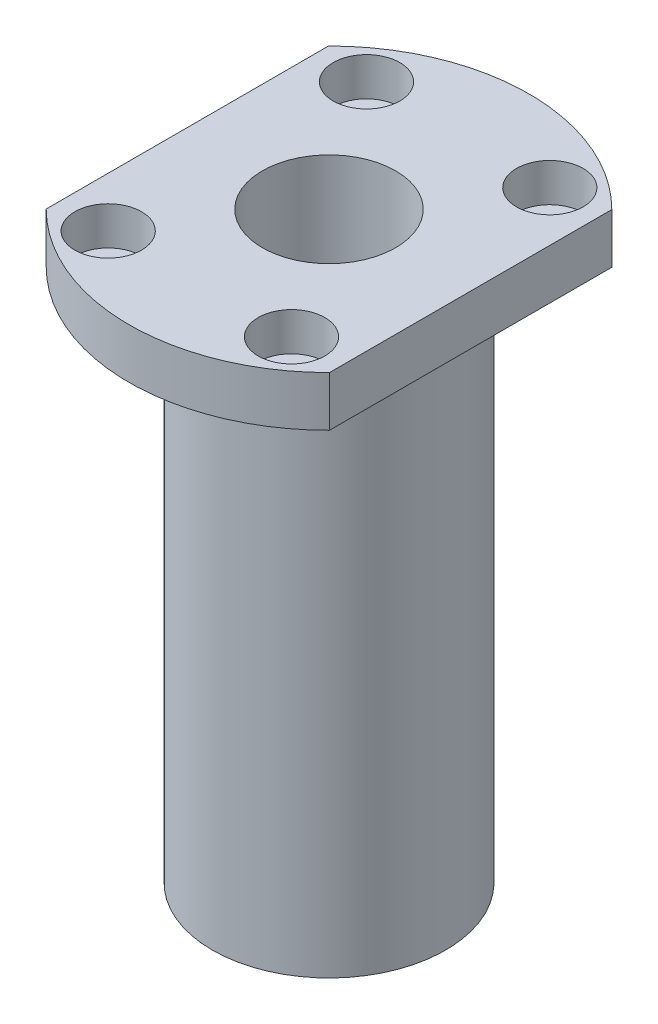
SolidWorks part; units mm, degrees
material "SS400"
ref_plane "Front Plane" through (0, 0, 0) normal (0, 0, 1) x (1, 0, 0)
ref_plane "Top Plane" through (0, 0, 0) normal (0, 1, 0) x (1, 0, 0)
ref_plane "Right Plane" through (0, 0, 0) normal (1, 0, 0) x (0, 0, -1)
sketch "Sketch1" plane through (0, 0, 0) normal (0, 1, 0) x (1, 0, 0)
  circle A0 centre (0, 0) radius 14
  dimension "D1" = 28
extrude "Boss-Extrude1" add sketch "Sketch1" along normal blind 64
sketch "Sketch2" plane through (0, 64, 0) normal (0, 1, 0) x (1, 0, 0)
  circle A0 centre (0, 0) radius 24
  dimension "D1" = 48
extrude "Boss-Extrude2" add sketch "Sketch2" along normal blind 6
sketch "Sketch3" plane through (0, 70, 0) normal (0, 1, 0) x (1, 0, 0)
  line L0 (0, 0) -> (0, 6.8507) construction
  line L1 (-17, 16.9411) -> (-17, -16.9411)
  line L2 (17, 16.9411) -> (17, -16.9411)
  arc A0 (17, 16.9411) -> (-17, 16.9411) centre (0, 0) ccw
  circle A1 centre (0, 0) radius 24
  arc A2 (-17, -16.9411) -> (17, -16.9411) centre (0, 0) ccw
  dimension "D1" = 0
  dimension "D2" = 34
extrude "Cut-Extrude2" cut sketch "Sketch3" against normal blind 6 flip side to cut
sketch "Sketch4" plane through (0, 0, 0) normal (0, -1, 0) x (1, 0, 0)
  circle A0 centre (0, 0) radius 8
  dimension "D1" = 16
extrude "Cut-Extrude3" cut sketch "Sketch4" against normal through all
hole_wizard "Hole size per socket head cap screw type1" positions "Sketch6" profile "Sketch5" counterbore size "M4" standard "GB" end condition through all
sketch "Sketch6" plane through (0, 70, 0) normal (0, 1, 0) x (-1, 0, 0)
  line L0 (0, 0) -> (0, 4.4514) construction
  line L2 (0, 0) -> (5.7458, 0) construction
  point P1 (-11, 15.5)
  point P12 (11, 15.5)
  point P13 (11, -15.5)
  point P14 (-11, -15.5)
  dimension "D1" = 22
  dimension "D2" = 31
sketch "Sketch5" plane through (11, 70, 15.5) normal (1, 0, 0) x (0, 0, 1)
  line L0 (0, 0) -> (0, 70)
  line L1 (0, 70) -> (2.25, 70)
  line L3 (2.25, 70) -> (2.25, 4.6)
  line L4 (2.25, 4.6) -> (4, 4.6)
  line L5 (4, 4.6) -> (4, 0)
  line L7 (4, 0) -> (0, 0)
  line L11 (0, -6.35) -> (0, 107.95) construction
  dimension "通孔孔直径" = 4.5
  dimension "通孔孔深度" = 70
  dimension "柱形沉头孔直径" = 8
  dimension "柱形沉头孔深度" = 4.6
